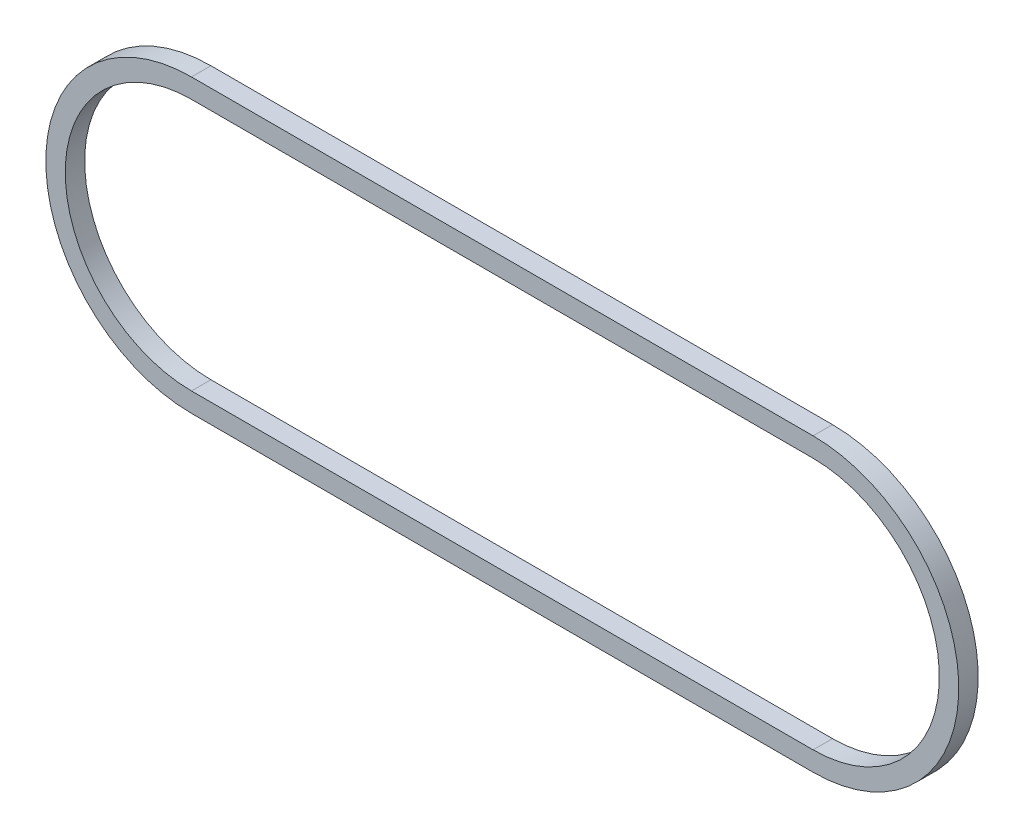
SolidWorks part; units mm, degrees
ref_plane "前视基准面" through (0, 0, 0) normal (0, 0, 1) x (1, 0, 0)
ref_plane "上视基准面" through (0, 0, 0) normal (0, 1, 0) x (1, 0, 0)
ref_plane "右视基准面" through (0, 0, 0) normal (1, 0, 0) x (0, 0, -1)
sketch "草图1" plane through (0, 0, 0) normal (0, 0, 1) x (1, 0, 0)
  line L0 (0, 0) -> (320, 0) construction
  line L1 (0, 75) -> (320, 75)
  line L2 (0, -75) -> (320, -75)
  line L3 (0, 65) -> (320, 65)
  line L4 (0, -65) -> (320, -65)
  arc A0 (0, 75) -> (0, -75) centre (0, 0) ccw
  arc A1 (320, -75) -> (320, 75) centre (320, 0) ccw
  arc A2 (320, -65) -> (320, 65) centre (320, 0) ccw
  arc A3 (0, 65) -> (0, -65) centre (0, 0) ccw
  point P3 (160, 0)
  dimension "D1" = 320
  dimension "D2" = 150
  dimension "D3" = 10
extrude "凸台-拉伸1" add sketch "草图1" along normal blind 10
